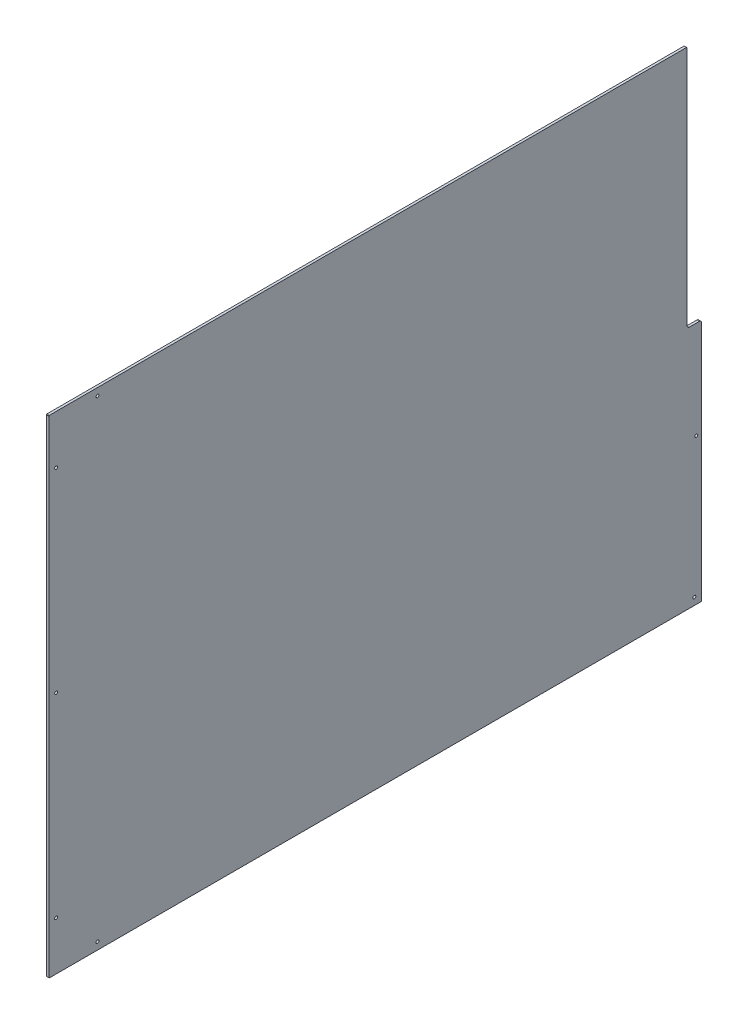
from build123d import *

# Parameters (mm, degrees)
SKETCH_1_W          = 1340
SKETCH_1_H          = 1000
EXTRUDE_1_DEPTH     = 5
CHAMFER_1_SIZE      = 1
SKETCH_2_R          = 3
CUT_EXTRUDE_1_DEPTH = 837.017344318
SKETCH_3_W          = 30
SKETCH_3_H          = 500
CUT_EXTRUDE_2_DEPTH = 10
CHAMFER_2_SIZE      = 1
FILLET_1_R          = 5
FILLET_2_R          = 5


with BuildPart() as part:
    # 草图1 → 凸台-拉伸1 (new body)
    with BuildSketch(Plane(origin=(0, 0, 0), x_dir=(0, 0, -1), z_dir=(1, 0, 0))):
        Rectangle(SKETCH_1_W, SKETCH_1_H)
    extrude(amount=EXTRUDE_1_DEPTH)

    # 倒角1
    chamfer_1_edges = [part.edges().sort_by_distance(p)[0] for p in [
        (2.5, 500, 670),
        (2.5, 500, -670),
        (2.5, -500, -670),
        (2.5, -500, 670),
    ]]
    chamfer(chamfer_1_edges, length=CHAMFER_1_SIZE)

    # 草图2 → 切除-拉伸1 (cut, through all)
    with BuildSketch(Plane.ZY):
        with Locations((-655, 485)):
            Circle(SKETCH_2_R)
        with Locations(Location((-655, -485, 0), (0, 0, 180))):
            Circle(SKETCH_2_R)
        with Locations((570, 485)):
            Circle(SKETCH_2_R)
        with Locations((655, 400)):
            Circle(SKETCH_2_R)
        with Locations((655, -400)):
            Circle(SKETCH_2_R)
        with Locations((570, -485)):
            Circle(SKETCH_2_R)
        with Locations((655, 0)):
            Circle(SKETCH_2_R)
        with Locations((-659, 200)):
            Circle(SKETCH_2_R)
        with Locations((-659, -200)):
            Circle(SKETCH_2_R)
    extrude(amount=-CUT_EXTRUDE_1_DEPTH, mode=Mode.SUBTRACT)

    # 草图3 → 切除-拉伸2 (cut)
    with BuildSketch(Plane(origin=(5, 0, 0), x_dir=(0, 0, -1), z_dir=(1, 0, 0))):
        with Locations((655, 250)):
            Rectangle(SKETCH_3_W, SKETCH_3_H)
    extrude(amount=-CUT_EXTRUDE_2_DEPTH, mode=Mode.SUBTRACT)

    # 倒角2
    chamfer_2_edges = [part.edges().sort_by_distance(p)[0] for p in [
        (2.5, 500, -640),
    ]]
    chamfer(chamfer_2_edges, length=CHAMFER_2_SIZE)

    # 圆角1
    fillet_1_edges = [part.edges().sort_by_distance(p)[0] for p in [
        (2.5, 0, -640),
    ]]
    fillet(fillet_1_edges, radius=FILLET_1_R)

    # 圆角2
    fillet_2_edges = [part.edges().sort_by_distance(p)[0] for p in [
        (2.5, 0, -670),
    ]]
    fillet(fillet_2_edges, radius=FILLET_2_R)


solid = part.part
